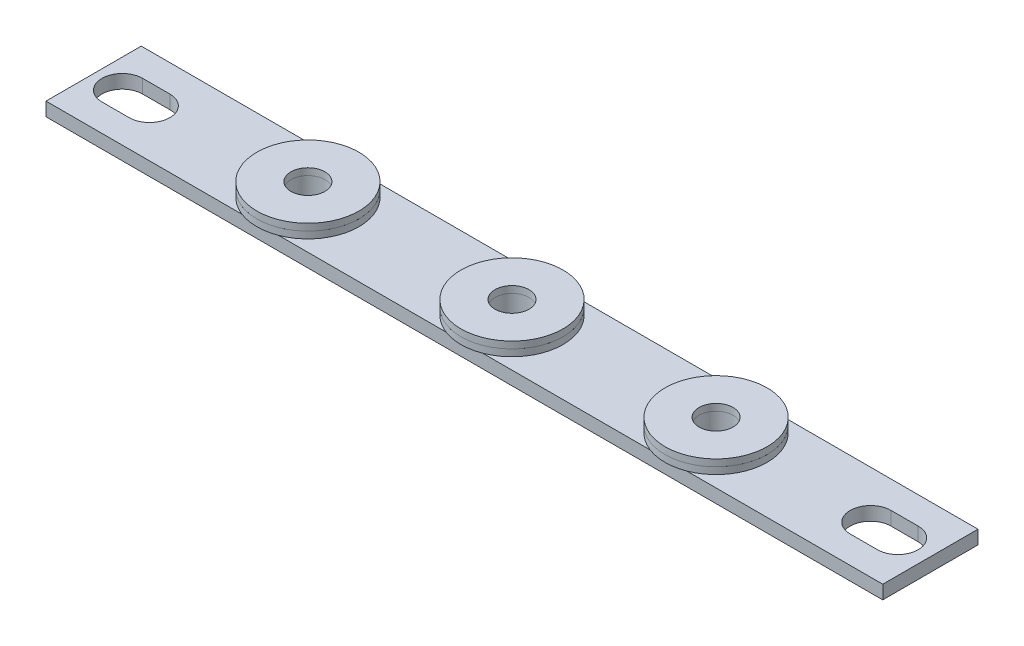
from build123d import *

# Parameters (mm, degrees)
SKETCH1_W             = 123
SKETCH1_H             = 14
SKETCH1_R             = 2.5
BOSS_EXTRUDE1_DEPTH   = 2
SKETCH2_R             = 7.5
SKETCH2_R_2           = 2.5
BOSS_EXTRUDE2_DEPTH   = 1
SKETCH3_R             = 7.5
SKETCH3_R_2           = 2.5
BOSS_EXTRUDE3_DEPTH   = 1
BOSS_EXTRUDE3_2_DEPTH = 1
BOSS_EXTRUDE3_3_DEPTH = 1


with BuildPart() as part:
    # Sketch1 → Boss-Extrude1 (new body)
    with BuildSketch(Plane(origin=(0, 0, 0), x_dir=(1, 0, 0), z_dir=(0, 1, 0))):
        Rectangle(SKETCH1_W, SKETCH1_H)
        with Locations(Location((-30, 0, 0), (0, 0, 270))):
            Circle(SKETCH1_R, mode=Mode.SUBTRACT)
        with Locations(Location((0, 0, 0), (0, 0, 270))):
            Circle(SKETCH1_R, mode=Mode.SUBTRACT)
        with Locations(Location((30, 0, 0), (0, 0, 270))):
            Circle(SKETCH1_R, mode=Mode.SUBTRACT)
        with BuildLine():
            Line((-57.285714286, 3), (-53.285714286, 3))
            ThreePointArc((-53.285714286, 3), (-50.285714286, 0), (-53.285714286, -3))
            Line((-53.285714286, -3), (-57.285714286, -3))
            ThreePointArc((-57.285714286, -3), (-60.285714286, 0), (-57.285714286, 3))
        make_face(mode=Mode.SUBTRACT)
        with BuildLine():
            Line((52.714285714, 3), (56.714285714, 3))
            ThreePointArc((56.714285714, 3), (59.714285714, 0), (56.714285714, -3))
            Line((56.714285714, -3), (52.714285714, -3))
            ThreePointArc((52.714285714, -3), (49.714285714, 0), (52.714285714, 3))
        make_face(mode=Mode.SUBTRACT)
    extrude(amount=BOSS_EXTRUDE1_DEPTH)

    # Sketch2 → Boss-Extrude2 (add)
    # profile 1 of 3: a face of its own
    with BuildSketch(Plane(origin=(0, 2, 0), x_dir=(1, 0, 0), z_dir=(0, 1, 0))):
        with Locations(Location((-30, 0, 0), (0, 0, 68.960530219))):
            Circle(SKETCH2_R)
        with Locations(Location((-30, 0, 0), (0, 0, 270))):
            Circle(SKETCH2_R_2, mode=Mode.SUBTRACT)
    # profile 2 of 3: a face of its own
    with BuildSketch(Plane(origin=(0, 2, 0), x_dir=(1, 0, 0), z_dir=(0, 1, 0))):
        with Locations(Location((0, 0, 0), (0, 0, 111.039469781))):
            Circle(SKETCH2_R)
        with Locations(Location((0, 0, 0), (0, 0, 270))):
            Circle(SKETCH2_R_2, mode=Mode.SUBTRACT)
    # profile 3 of 3: a face of its own
    with BuildSketch(Plane(origin=(0, 2, 0), x_dir=(1, 0, 0), z_dir=(0, 1, 0))):
        with Locations(Location((30, 0, 0), (0, 0, 68.960530219))):
            Circle(SKETCH2_R)
        with Locations(Location((30, 0, 0), (0, 0, 270))):
            Circle(SKETCH2_R_2, mode=Mode.SUBTRACT)
    extrude(amount=BOSS_EXTRUDE2_DEPTH)


with BuildPart() as body_2:
    # Sketch3 → Boss-Extrude3 (new body)
    with BuildSketch(Plane(origin=(0, 3, 0), x_dir=(1, 0, 0), z_dir=(0, 1, 0))):
        with Locations(Location((-30, 0, 0), (0, 0, 270))):
            Circle(SKETCH3_R)
        with Locations(Location((-30, 0, 0), (0, 0, 270))):
            Circle(SKETCH3_R_2, mode=Mode.SUBTRACT)
    extrude(amount=BOSS_EXTRUDE3_DEPTH)


with BuildPart() as body_3:
    # Sketch3 → Boss-Extrude3 2 (new body)
    with BuildSketch(Plane(origin=(0, 3, 0), x_dir=(1, 0, 0), z_dir=(0, 1, 0))):
        with Locations(Location((0, 0, 0), (0, 0, 270))):
            Circle(SKETCH3_R)
        with Locations(Location((0, 0, 0), (0, 0, 270))):
            Circle(SKETCH3_R_2, mode=Mode.SUBTRACT)
    extrude(amount=BOSS_EXTRUDE3_2_DEPTH)


with BuildPart() as body_4:
    # Sketch3 → Boss-Extrude3 3 (new body)
    with BuildSketch(Plane(origin=(0, 3, 0), x_dir=(1, 0, 0), z_dir=(0, 1, 0))):
        with Locations(Location((30, 0, 0), (0, 0, 270))):
            Circle(SKETCH3_R)
        with Locations(Location((30, 0, 0), (0, 0, 270))):
            Circle(SKETCH3_R_2, mode=Mode.SUBTRACT)
    extrude(amount=BOSS_EXTRUDE3_3_DEPTH)


solid = Compound([part.part, body_2.part, body_3.part, body_4.part])
